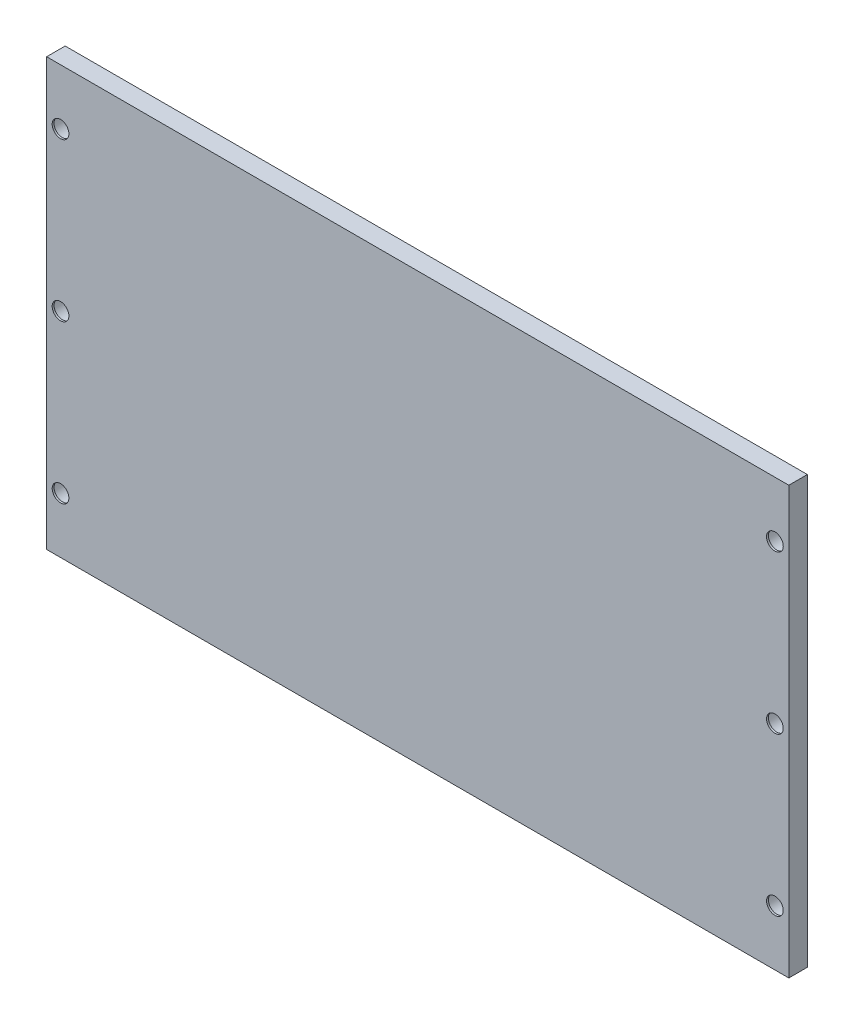
from build123d import *

# Parameters (mm, degrees)
SKETCH1_W           = 400
SKETCH1_H           = 230
BOSS_EXTRUDE1_DEPTH = 10
SKETCH2_R           = 4.5
CUT_EXTRUDE1_DEPTH  = 25
SKETCH3_R           = 6.5
CUT_EXTRUDE2_DEPTH  = 9


with BuildPart() as part:
    # Sketch1 → Boss-Extrude1 (new body)
    with BuildSketch(Plane.XY):
        Rectangle(SKETCH1_W, SKETCH1_H)
    extrude(amount=BOSS_EXTRUDE1_DEPTH)

    # Sketch2 → Cut-Extrude1 (cut)
    with BuildSketch(Plane(origin=(0, 0, 0), x_dir=(-1, 0, 0), z_dir=(0, 0, -1))):
        with Locations((192.5, -85)):
            Circle(SKETCH2_R)
        with Locations((192.5, 0)):
            Circle(SKETCH2_R)
        with Locations((192.5, 85)):
            Circle(SKETCH2_R)
    cut_extrude1 = extrude(amount=-CUT_EXTRUDE1_DEPTH, mode=Mode.SUBTRACT)

    # Sketch3 → Cut-Extrude2 (cut)
    with BuildSketch(Plane(origin=(0, 0, 0), x_dir=(-1, 0, 0), z_dir=(0, 0, -1))):
        with Locations((192.5, -85)):
            Circle(SKETCH3_R)
        with Locations((192.5, 0)):
            Circle(SKETCH3_R)
        with Locations((192.5, 85)):
            Circle(SKETCH3_R)
    cut_extrude2 = extrude(amount=-CUT_EXTRUDE2_DEPTH, mode=Mode.SUBTRACT)

    # Mirror1: Cut-Extrude1, Cut-Extrude2 across plane
    add(cut_extrude1.mirror(Plane(origin=(0, 0, 0), x_dir=(0, 0, 1), z_dir=(1, 0, 0))), mode=Mode.SUBTRACT)
    add(cut_extrude2.mirror(Plane(origin=(0, 0, 0), x_dir=(0, 0, 1), z_dir=(1, 0, 0))), mode=Mode.SUBTRACT)


solid = part.part
